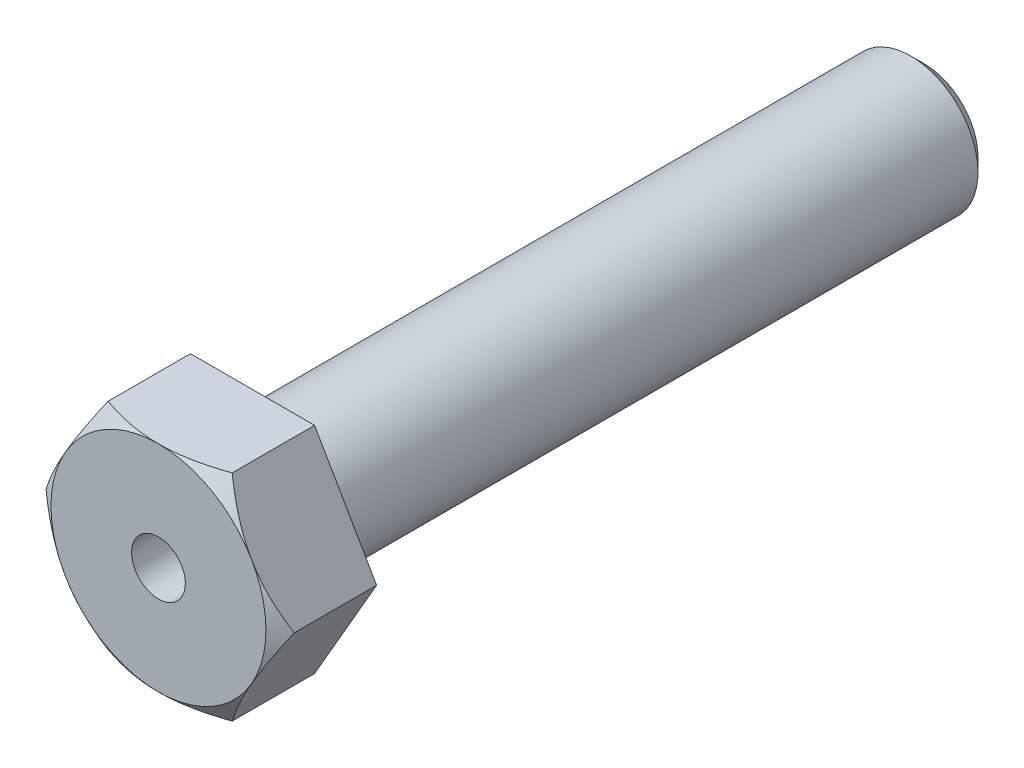
from build123d import *

# Parameters (mm, degrees)
BOSS_EXTRUDE1_START = -3.5
SKETCH4_R           = 1
BOSS_EXTRUDE1_DEPTH = 3.5
SKETCH5_R           = 5.237604307
SKETCH5_R_2         = 4
CUT_EXTRUDE1_DEPTH  = 1
CUT_EXTRUDE1_DRAFT  = -55
CHAMFER1_SIZE       = 0.5


with BuildPart() as part:
    # Sketch3 → Revolve1 (revolve)
    with BuildSketch(Plane(origin=(0, 0, 0), x_dir=(0, 0, -1), z_dir=(1, 0, 0)), mode=Mode.PRIVATE) as revolve1_sk:
        Polygon((0, 2.5), (-3.5, 2.5), (-3.5, 1), (25, 1), (25, 2.5), align=None)
    revolve(revolve1_sk.sketch.rotate(Axis((0, 0, 3.5), (0, 0, -1)), 180), axis=Axis((0, 0, 3.5), (0, 0, -1)))

    # Sketch4 → Boss-Extrude1 (add)
    with BuildSketch(Plane.XY.offset(3.5).offset(BOSS_EXTRUDE1_START)):
        Polygon((2.309401077, 4), (-2.309401077, 4), (-4.618802154, 0), (-2.309401077, -4), (2.309401077, -4), (4.618802154, 0), align=None)
        with Locations(Location((0, 0, 0), (0, 0, 270))):
            Circle(SKETCH4_R, mode=Mode.SUBTRACT)
    extrude(amount=BOSS_EXTRUDE1_DEPTH)


with BuildPart() as cut_extrude1_tool:
    # Sketch5 → Cut-Extrude1 (with draft: the straight prism first)
    with BuildSketch(Plane.XY.offset(3.5)):
        Circle(SKETCH5_R)
        Circle(SKETCH5_R_2, mode=Mode.SUBTRACT)
    extrude(amount=-CUT_EXTRUDE1_DEPTH)
    # Cut-Extrude1: the draft: its side faces are tilted about the plane it starts from
    cut_extrude1_sides = [cut_extrude1_tool.faces().sort_by_distance(p)[0] for p in [
        (-5.237604307, 0, 3),
        (-4, 0, 3),
    ]]
    draft(cut_extrude1_sides, Plane.XY.offset(3.5), CUT_EXTRUDE1_DRAFT)


with BuildPart() as part_1:
    add(part.part)

    # Cut-Extrude1: cut by cut_extrude1_tool
    add(cut_extrude1_tool.part, mode=Mode.SUBTRACT)

    # Chamfer1
    chamfer1_edges = [part_1.edges().sort_by_distance(p)[0] for p in [
        (0, 2.5, -25),
    ]]
    chamfer(chamfer1_edges, length=CHAMFER1_SIZE)


solid = part_1.part
